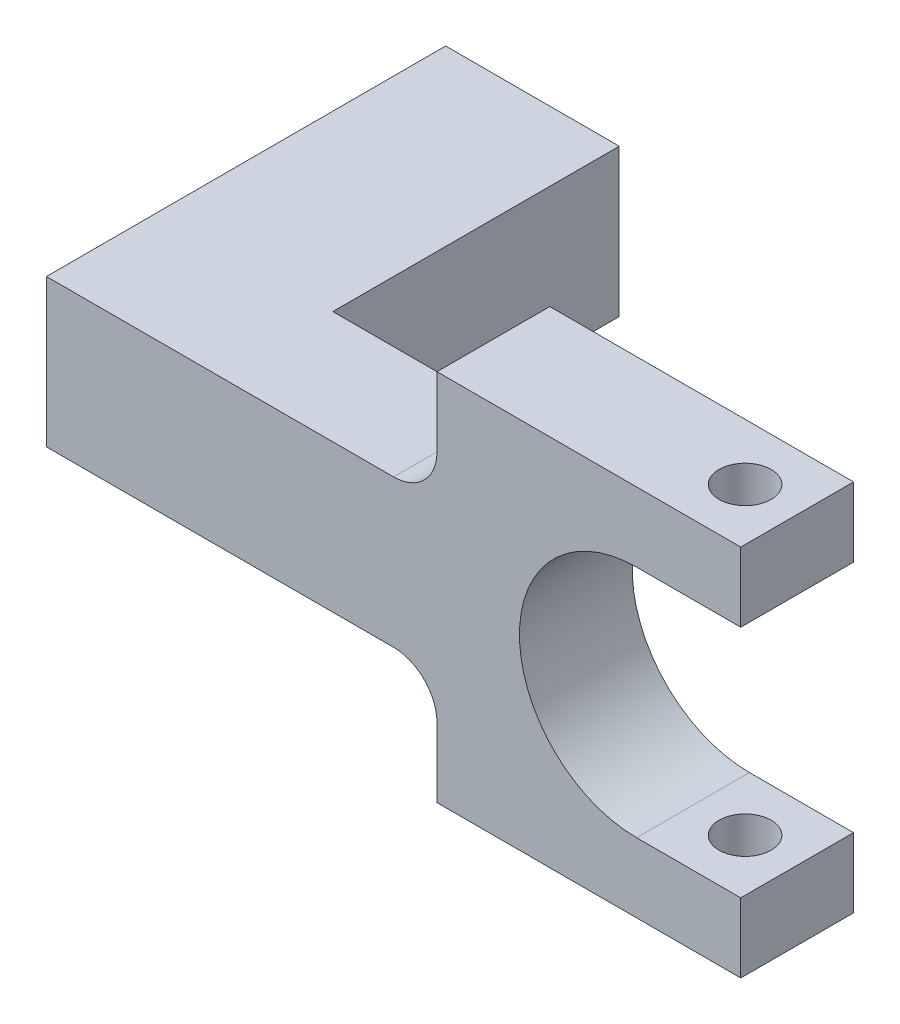
SolidWorks part; units mm, degrees
ref_plane "前视基准面" through (0, 0, 0) normal (0, 0, 1) x (1, 0, 0)
ref_plane "上视基准面" through (0, 0, 0) normal (0, 1, 0) x (1, 0, 0)
ref_plane "右视基准面" through (0, 0, 0) normal (1, 0, 0) x (0, 0, -1)
sketch "草图1" plane through (0, 0, 0) normal (0, 0, 1) x (1, 0, 0)
  line L0 (0, 13.5) -> (12, 13.5)
  line L1 (12, 13.5) -> (12, 21.5)
  line L2 (12, 21.5) -> (-68, 21.5)
  line L3 (-68, 21.5) -> (-68, -21.5)
  line L4 (-68, -21.5) -> (12, -21.5)
  line L5 (12, -21.5) -> (12, -13.5)
  line L6 (12, -13.5) -> (0, -13.5)
  arc A0 (0, 13.5) -> (0, -13.5) centre (0, 0) ccw
  dimension "D1" = 13.5
  dimension "D2" = 12
  dimension "D3" = 8
  dimension "D4" = 80
extrude "凸台-拉伸1" add sketch "草图1" along normal mid plane 13
sketch "草图2" plane through (0, 0, 6.5) normal (0, 0, 1) x (1, 0, 0)
  line L1 (-68, 21.5) -> (-23, 21.5)
  line L2 (-68, 21.5) -> (-68, 8.5)
  line L3 (-68, 8.5) -> (-23, 8.5)
  line L4 (-23, 21.5) -> (-23, 8.5)
  line L5 (-68, -21.5) -> (-23, -21.5)
  line L6 (-68, -21.5) -> (-68, -8.5)
  line L7 (-68, -8.5) -> (-23, -8.5)
  line L8 (-23, -21.5) -> (-23, -8.5)
  dimension "D1" = 45
  dimension "D2" = 13
extrude "切除-拉伸1" cut sketch "草图2" against normal up to next
fillet "圆角1" radius 5 2 edges at (-23, -8.5, 0) (-23, 8.5, 0)
sketch "草图3" plane through (0, 0, -6.5) normal (0, 0, -1) x (-1, 0, 0)
  line L1 (68, -8.5) -> (48, -8.5)
  line L2 (68, -8.5) -> (68, 8.5)
  line L3 (68, 8.5) -> (48, 8.5)
  line L4 (48, -8.5) -> (48, 8.5)
  line L5 (28, 8.5) -> (68, 8.5) construction
  dimension "D1" = 20
extrude "凸台-拉伸2" add sketch "草图3" along normal blind 33
sketch "草图4" plane through (0, -21.5, 0) normal (0, -1, 0) x (1, 0, 0)
  line L0 (12, 6.5) -> (12, -6.5) construction
  circle A0 centre (6, 0) radius 3
  dimension "D1" = 6
  dimension "D2" = 6
extrude "切除-拉伸2" cut sketch "草图4" against normal up to surface (43 mm away) up to face at (-5.5, 21.5, 0)
